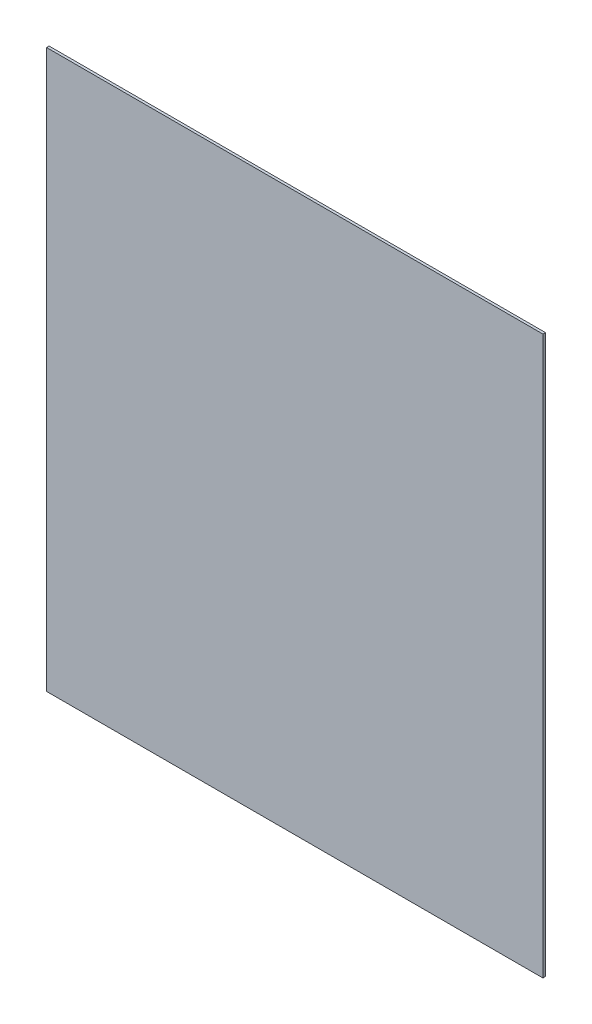
SolidWorks part; units mm, degrees
material "PMMA(有机玻璃)"
ref_plane "前视" through (0, 0, 0) normal (0, 0, 1) x (1, 0, 0)
ref_plane "上视" through (0, 0, 0) normal (0, 1, 0) x (1, 0, 0)
ref_plane "右视" through (0, 0, 0) normal (1, 0, 0) x (0, 0, -1)
sketch "草图1" plane through (0, 0, 0) normal (0, 0, 1) x (1, 0, 0)
  line L1 (-486, 546) -> (486, 546)
  line L2 (-486, 546) -> (-486, -546)
  line L3 (-486, -546) -> (486, -546)
  line L4 (486, 546) -> (486, -546)
  line L5 (-486, 546) -> (486, -546) construction
  line L6 (-486, -546) -> (486, 546) construction
  point P0 (0, 0)
  dimension "D1" = 1092
  dimension "D2" = 972
extrude "凸台-拉伸1" add sketch "草图1" along normal blind 5
hole_wizard "M5 间隙孔1" positions "草图3" profile "草图2" hole size "M5" standard "GB"
sketch "草图3" plane through (0, 0, 5) normal (0, 0, 1) x (1, 0, 0)
  line L0 (-427.5, 273) -> (-427.5, -273) construction
  line L1 (-427.5, -273) -> (427.5, -273) construction
  line L2 (0, 273) -> (0, -273) construction
  line L3 (427.5, 273) -> (-427.5, 273) construction
  line L5 (-427.5, 0) -> (427.5, 0) construction
  line L6 (427.5, -273) -> (427.5, 273) construction
  point P0 (-375, -261)
  point P46 (415.5, 250)
  point P48 (-415.5, 250)
  point P58 (-125, -261)
  point P59 (125, -261)
  point P61 (-125, 261)
  point P62 (125, 261)
  point P64 (-375, 261)
  point P88 (375, -261)
  point P89 (375, 261)
  point P108 (415.5, 0)
  point P109 (-415.5, 0)
  point P110 (415.5, -250)
  point P111 (-415.5, -250)
  dimension "D1" = 12
  dimension "D2" = 12
  dimension "D5" = 3
  dimension "D3" = 12
  dimension "D6" = 4
  dimension "D4" = 2
sketch "草图2" plane through (-375, -261, 5) normal (1, 0, 0) x (0, -1, 0)
  line L0 (0, 0) -> (0, 5)
  line L1 (0, 5) -> (2.75, 5)
  line L2 (2.75, 5) -> (2.75, 0)
  line L5 (2.75, 0) -> (0, 0)
  line L11 (0, -6.35) -> (0, 107.95) construction
  dimension "通孔孔直径" = 5.5
  dimension "通孔孔深度" = 5
